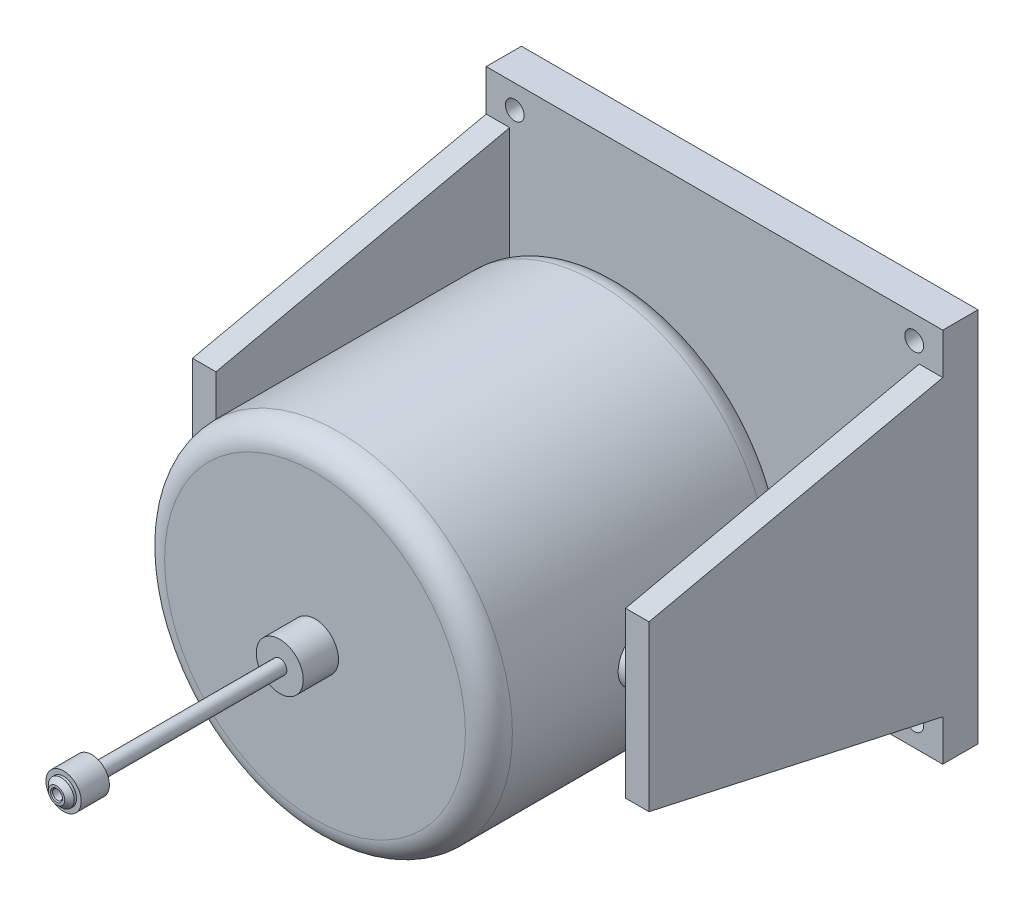
SolidWorks part; units mm, degrees
material "软铁(SN)"
ref_plane "Front Plane" through (0, 0, 0) normal (0, 0, 1) x (1, 0, 0)
ref_plane "Top Plane" through (0, 0, 0) normal (0, 1, 0) x (1, 0, 0)
ref_plane "Right Plane" through (0, 0, 0) normal (1, 0, 0) x (0, 0, -1)
sketch "Sketch1" plane through (0, 0, 0) normal (0, 0, 1) x (1, 0, 0)
  circle A0 centre (0, 0) radius 74
  dimension "D1" = 148
extrude "Boss-Extrude1" add sketch "Sketch1" along normal mid plane 130
fillet "Fillet1" radius 10 2 edges at (74, 0, -65) (74, 0, 65)
sketch "Sketch2" plane through (0, 0, 65) normal (0, 0, 1) x (1, 0, 0)
  circle A0 centre (0, 0) radius 10
  dimension "D1" = 20
extrude "Boss-Extrude2" add sketch "Sketch2" along normal blind 15
sketch "Sketch3" plane through (0, 0, 80) normal (0, 0, 1) x (1, 0, 0)
  line L1 (97.1429, -80) -> (-97.1429, -80)
  line L2 (97.1429, -80) -> (97.1429, 80)
  line L3 (97.1429, 80) -> (-97.1429, 80)
  line L4 (-97.1429, -80) -> (-97.1429, 80)
  line L5 (97.1429, -80) -> (-97.1429, 80) construction
  line L6 (97.1429, 80) -> (-97.1429, -80) construction
  circle A0 centre (-85, 70) radius 4
  circle A1 centre (85, 70) radius 4
  circle A2 centre (85, -70) radius 4
  circle A3 centre (-85, -70) radius 4
  point P0 (0, 0)
  dimension "D1" = 8
  dimension "D2" = 170
  dimension "D3" = 140
  dimension "D4" = 10
extrude "Boss-Extrude3" add sketch "Sketch3" along normal blind 15 from offset 200 separate body offset against normal yes
sketch "Sketch4" plane through (-97.1429, 0, 0) normal (-1, 0, 0) x (0, 0, 1)
  line L0 (-105, 62.5) -> (20, 35)
  line L1 (-105, 80) -> (-105, -80) construction
  line L2 (20, 35) -> (20, -35)
  line L3 (20, -35) -> (-105, -62.5)
  line L4 (-105, -62.5) -> (-105, 62.5)
  line L5 (0, 0) -> (-50000, 0) construction
  dimension "D1" = 125
  dimension "D2" = 70
  dimension "D3" = 20
extrude "Boss-Extrude4" add sketch "Sketch4" against normal blind 10
mirror "Mirror1" about plane through (0, 0, 0) normal (1, 0, 0) of "Boss-Extrude4"
sketch "Sketch5" plane through (0, 0, 0) normal (1, 0, 0) x (0, 0, -1)
  circle A0 centre (0, 0) radius 10
  dimension "D1" = 20
extrude "Boss-Extrude5" add sketch "Sketch5" along normal mid plane 180
sketch "Sketch6" plane through (0, 0, 80) normal (0, 0, 1) x (1, 0, 0)
  circle A0 centre (0, 0) radius 3
  dimension "D1" = 6
extrude "Boss-Extrude6" add sketch "Sketch6" along normal blind 80
sketch "Sketch7" plane through (0, 0, 160) normal (0, 0, 1) x (1, 0, 0)
  circle A0 centre (0, 0) radius 7.5
  dimension "D1" = 15
extrude "Boss-Extrude7" add sketch "Sketch7" along normal blind 12
sketch "Sketch8" plane through (0, 0, 172) normal (0, 0, 1) x (1, 0, 0)
  circle A0 centre (0, 0) radius 5.5
  dimension "D1" = 11
extrude "Boss-Extrude8" add sketch "Sketch8" along normal blind 3
chamfer "Chamfer1" distance 2 angle 45 1 edges at (5.5, 0, 175)
hole_wizard "M5 Tapped Hole1" positions "Sketch9" profile "Sketch10" tap size "M5" standard "GB"
sketch "Sketch9" plane through (0, 0, 175) normal (0, 0, 1) x (1, 0, 0)
  point P0 (0, 0)
sketch "Sketch10" plane through (0, 0, 175) normal (1, 0, 0) x (0, -1, 0)
  line L0 (0, 0) -> (0, 15.2618)
  line L1 (0, 15.2618) -> (2.1, 14)
  line L2 (2.1, 14) -> (2.1, 0.425)
  line L3 (2.1, 0.425) -> (2.525, 0)
  line L5 (2.525, 0) -> (0, 0)
  line L6 (-2.1, 0.425) -> (-2.525, 0) construction
  line L10 (0, 15.2618) -> (-2.1, 14) construction
  line L11 (0, -6.35) -> (0, 107.95) construction
  dimension "螺纹孔钻头直径" = 4.2
  dimension "螺纹孔钻头深度" = 14
  dimension "近端锥形沉头孔直径" = 5.05
  dimension "近端锥形沉头孔角度" = 90
  dimension "导头角度" = 118
cosmetic thread "Cosmetic Thread1" parameters "D1"=10, "D2"=5
